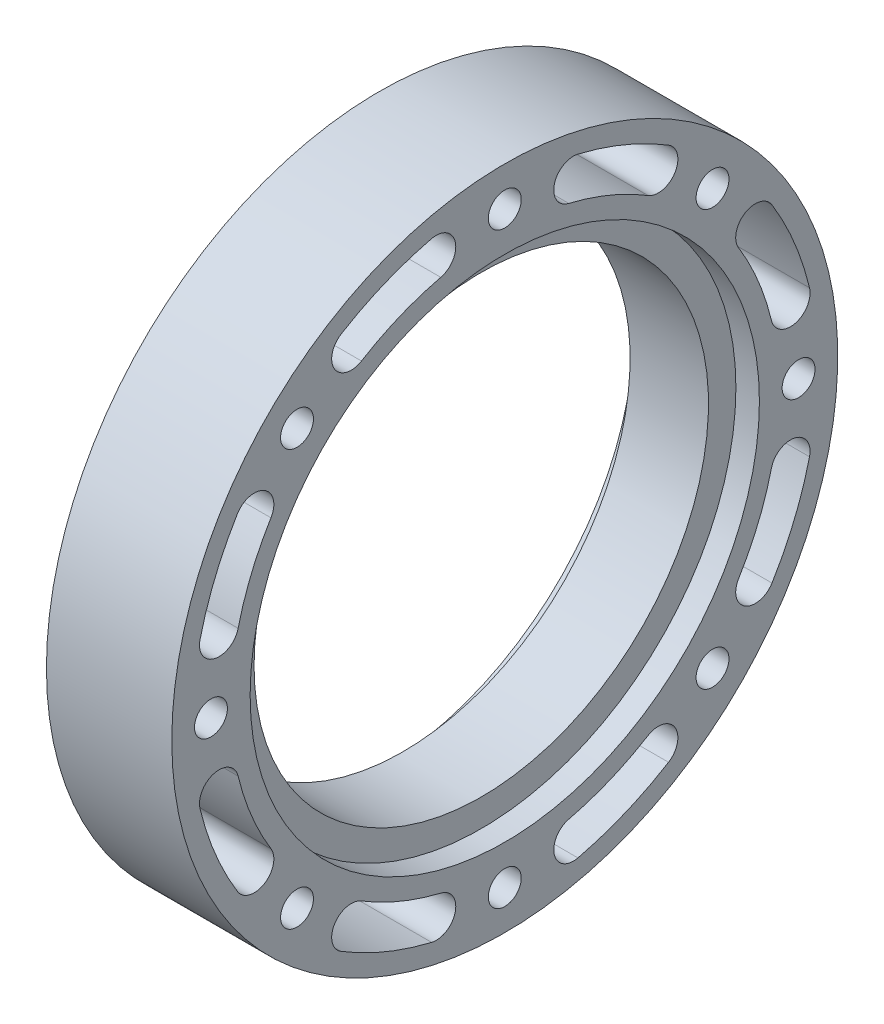
from build123d import *

# Parameters (mm, degrees)
SKETCH_2_R          = 2.1
CUT_EXTRUDE_1_DEPTH = 63.197266821


with BuildPart() as part:
    # 草图1 → 旋转1 (revolve)
    with BuildSketch(Plane(origin=(0, 0, 0), x_dir=(1, 0, 0), z_dir=(0, 1, 0)), mode=Mode.PRIVATE) as revolve_1_sk:
        Polygon((-5, 29), (-5, 32.5), (-8, 32.5), (-8, 42.5), (8, 42.5), (8, 32.5), (5, 32.5), (5, 29), align=None)
    revolve(revolve_1_sk.sketch.rotate(Axis((-880.62625216, 0, 0), (1, 0, 0)), 180), axis=Axis((-880.62625216, 0, 0), (1, 0, 0)))

    # 草图2 → 切除-拉伸1 (cut, through all)
    with BuildSketch(Plane(origin=(8, 0, 0), x_dir=(0, 0, -1), z_dir=(1, 0, 0))):
        with Locations((0, 37.5)):
            Circle(SKETCH_2_R)
        with Locations((26.516504294, 26.516504294)):
            Circle(SKETCH_2_R)
        with Locations((37.5, 0)):
            Circle(SKETCH_2_R)
        with Locations((26.516504294, -26.516504294)):
            Circle(SKETCH_2_R)
        with Locations((0, -37.5)):
            Circle(SKETCH_2_R)
        with Locations((-26.516504294, -26.516504294)):
            Circle(SKETCH_2_R)
        with Locations((-37.5, 0)):
            Circle(SKETCH_2_R)
        with Locations((-26.516504294, 26.516504294)):
            Circle(SKETCH_2_R)
        with BuildLine():
            ThreePointArc((20.899942589, 34.105606574), (15.307337295, 36.9551813), (9.337814554, 38.894796816))
            ThreePointArc((9.337814554, 38.894796816), (6.323276344, 37.047485425), (8.170587735, 34.032947214))
            ThreePointArc((8.170587735, 34.032947214), (13.393920133, 32.335783638), (18.287449765, 29.842405752))
            ThreePointArc((18.287449765, 29.842405752), (21.725296588, 30.667759751), (20.899942589, 34.105606574))
        make_face()
        with BuildLine():
            ThreePointArc((38.894796816, 9.337814554), (36.9551813, 15.307337295), (34.105606574, 20.899942589))
            ThreePointArc((34.105606574, 20.899942589), (30.667759751, 21.725296588), (29.842405752, 18.287449765))
            ThreePointArc((29.842405752, 18.287449765), (32.335783638, 13.393920133), (34.032947214, 8.170587735))
            ThreePointArc((34.032947214, 8.170587735), (37.047485425, 6.323276344), (38.894796816, 9.337814554))
        make_face()
        with BuildLine():
            ThreePointArc((34.105606574, -20.899942589), (36.9551813, -15.307337295), (38.894796816, -9.337814554))
            ThreePointArc((38.894796816, -9.337814554), (37.047485425, -6.323276344), (34.032947214, -8.170587735))
            ThreePointArc((34.032947214, -8.170587735), (32.335783638, -13.393920133), (29.842405752, -18.287449765))
            ThreePointArc((29.842405752, -18.287449765), (30.667759751, -21.725296588), (34.105606574, -20.899942589))
        make_face()
        with BuildLine():
            ThreePointArc((9.337814554, -38.894796816), (15.307337295, -36.9551813), (20.899942589, -34.105606574))
            ThreePointArc((20.899942589, -34.105606574), (21.725296588, -30.667759751), (18.287449765, -29.842405752))
            ThreePointArc((18.287449765, -29.842405752), (13.393920133, -32.335783638), (8.170587735, -34.032947214))
            ThreePointArc((8.170587735, -34.032947214), (6.323276344, -37.047485425), (9.337814554, -38.894796816))
        make_face()
        with BuildLine():
            ThreePointArc((-20.899942589, -34.105606574), (-15.307337295, -36.9551813), (-9.337814554, -38.894796816))
            ThreePointArc((-9.337814554, -38.894796816), (-6.323276344, -37.047485425), (-8.170587735, -34.032947214))
            ThreePointArc((-8.170587735, -34.032947214), (-13.393920133, -32.335783638), (-18.287449765, -29.842405752))
            ThreePointArc((-18.287449765, -29.842405752), (-21.725296588, -30.667759751), (-20.899942589, -34.105606574))
        make_face()
        with BuildLine():
            ThreePointArc((-38.894796816, -9.337814554), (-36.9551813, -15.307337295), (-34.105606574, -20.899942589))
            ThreePointArc((-34.105606574, -20.899942589), (-30.667759751, -21.725296588), (-29.842405752, -18.287449765))
            ThreePointArc((-29.842405752, -18.287449765), (-32.335783638, -13.393920133), (-34.032947214, -8.170587735))
            ThreePointArc((-34.032947214, -8.170587735), (-37.047485425, -6.323276344), (-38.894796816, -9.337814554))
        make_face()
        with BuildLine():
            ThreePointArc((-34.105606574, 20.899942589), (-36.9551813, 15.307337295), (-38.894796816, 9.337814554))
            ThreePointArc((-38.894796816, 9.337814554), (-37.047485425, 6.323276344), (-34.032947214, 8.170587735))
            ThreePointArc((-34.032947214, 8.170587735), (-32.335783638, 13.393920133), (-29.842405752, 18.287449765))
            ThreePointArc((-29.842405752, 18.287449765), (-30.667759751, 21.725296588), (-34.105606574, 20.899942589))
        make_face()
        with BuildLine():
            ThreePointArc((-9.337814554, 38.894796816), (-15.307337295, 36.9551813), (-20.899942589, 34.105606574))
            ThreePointArc((-20.899942589, 34.105606574), (-21.725296588, 30.667759751), (-18.287449765, 29.842405752))
            ThreePointArc((-18.287449765, 29.842405752), (-13.393920133, 32.335783638), (-8.170587735, 34.032947214))
            ThreePointArc((-8.170587735, 34.032947214), (-6.323276344, 37.047485425), (-9.337814554, 38.894796816))
        make_face()
    extrude(amount=-CUT_EXTRUDE_1_DEPTH, mode=Mode.SUBTRACT)


solid = part.part
